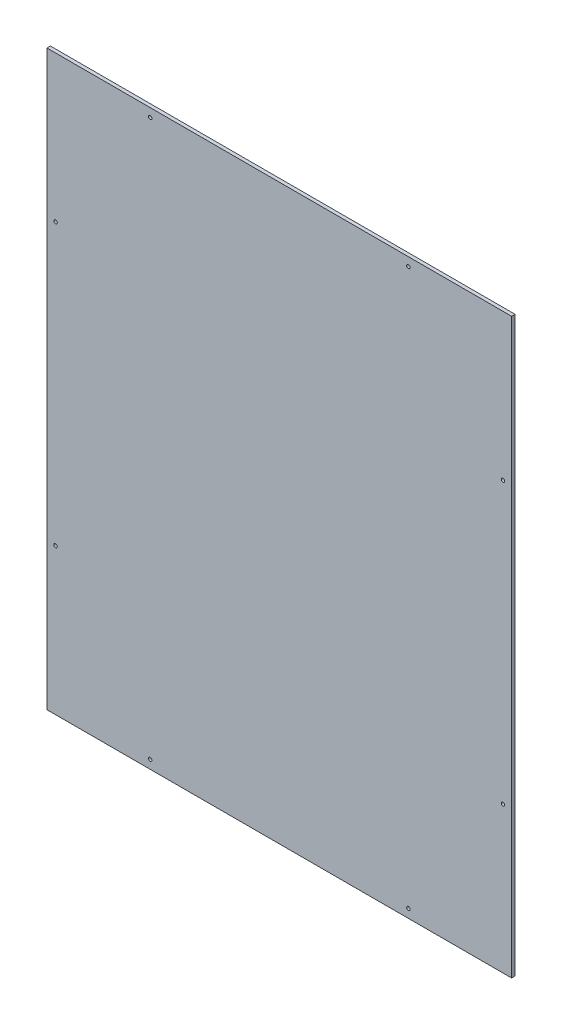
SolidWorks part; units mm, degrees
ref_plane "前视基准面" through (0, 0, 0) normal (0, 0, 1) x (1, 0, 0)
ref_plane "上视基准面" through (0, 0, 0) normal (0, 1, 0) x (1, 0, 0)
ref_plane "右视基准面" through (0, 0, 0) normal (1, 0, 0) x (0, 0, -1)
sketch "草图1" plane through (0, 0, 0) normal (0, 0, 1) x (1, 0, 0)
  line L1 (-270, -333) -> (270, -333)
  line L2 (-270, -333) -> (-270, 333)
  line L3 (-270, 333) -> (270, 333)
  line L4 (270, -333) -> (270, 333)
  line L5 (-270, -333) -> (270, 333) construction
  line L6 (-270, 333) -> (270, -333) construction
  point P0 (0, 0)
  dimension "D1" = 540
  dimension "D2" = 666
extrude "凸台-拉伸1" add sketch "草图1" along normal mid plane 4
hole_wizard "Ø4.0 (4) 直径孔1" positions "草图2" profile "草图3" hole size "Ø4.0" standard "GB" end condition through all
sketch "草图2" plane through (0, 0, -2) normal (0, 0, -1) x (-1, 0, 0)
  line L0 (-270, -333) -> (-270, 333) construction
  line L1 (-270, 333) -> (270, 333) construction
  line L2 (270, -333) -> (-270, -333) construction
  point P0 (-260, 163)
  point P2 (-260, -163)
  dimension "D1" = 10
  dimension "D2" = 170
  dimension "D3" = 170
  dimension "D4" = 10
sketch "草图3" plane through (260, 163, -2) normal (1, 0, 0) x (0, 1, 0)
  line L0 (0, 0) -> (0, 4)
  line L1 (0, 4) -> (2, 4)
  line L2 (2, 4) -> (2, 0)
  line L5 (2, 0) -> (0, 0)
  line L11 (0, -6.35) -> (0, 107.95) construction
  dimension "通孔孔直径" = 4
  dimension "通孔孔深度" = 4
hole_wizard "Ø4.0 (4) 直径孔2" positions "草图4" profile "草图5" hole size "Ø4.0" standard "GB" end condition through all
sketch "草图4" plane through (0, 0, -2) normal (0, 0, -1) x (-1, 0, 0)
  line L0 (-270, 333) -> (270, 333) construction
  line L1 (-270, -333) -> (-270, 333) construction
  line L2 (270, 333) -> (270, -333) construction
  point P0 (-150, 323)
  point P2 (150, 323)
  dimension "D1" = 10
  dimension "D2" = 120
  dimension "D3" = 120
  dimension "D4" = 10
sketch "草图5" plane through (150, 323, -2) normal (1, 0, 0) x (0, 1, 0)
  line L0 (0, 0) -> (0, 4)
  line L1 (0, 4) -> (2, 4)
  line L2 (2, 4) -> (2, 0)
  line L5 (2, 0) -> (0, 0)
  line L11 (0, -6.35) -> (0, 107.95) construction
  dimension "通孔孔直径" = 4
  dimension "通孔孔深度" = 4
mirror "镜向1" about plane through (0, 0, 0) normal (0, 1, 0) of "Ø4.0 (4) 直径孔2"
mirror "镜向2" about plane through (0, 0, 0) normal (1, 0, 0) of "Ø4.0 (4) 直径孔1"
